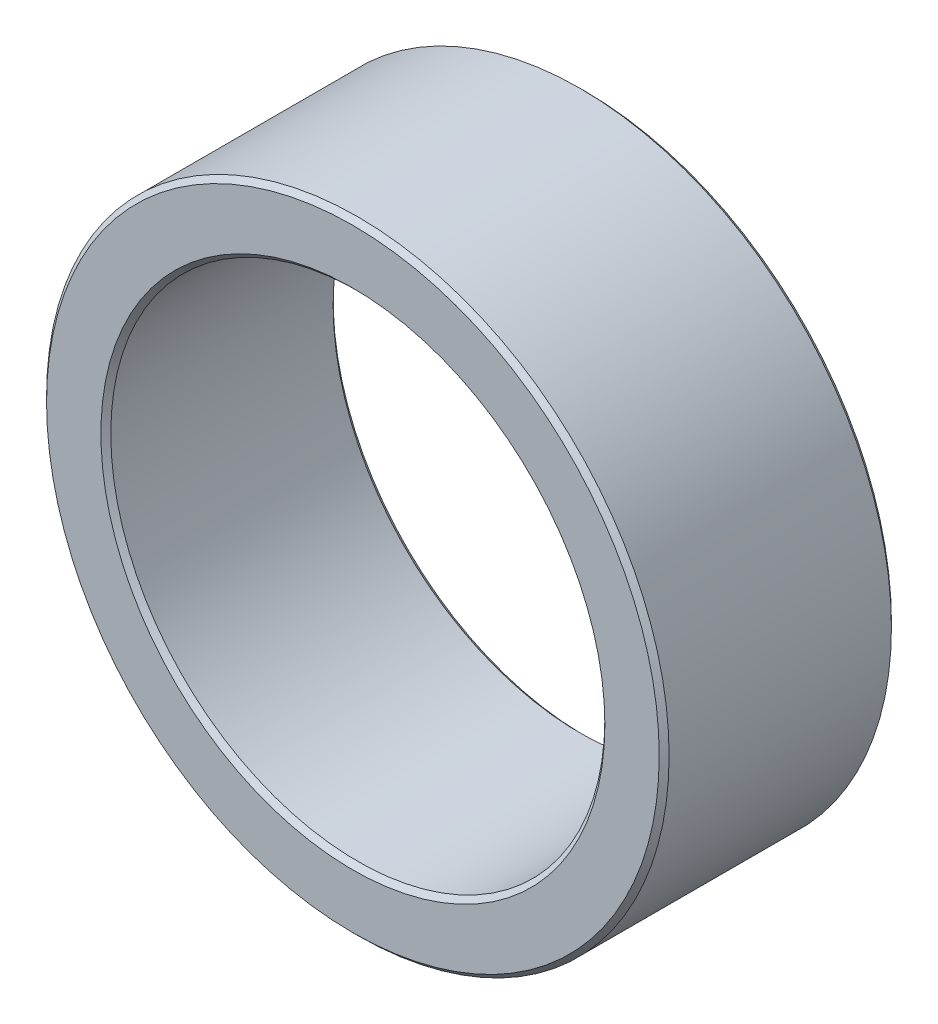
from build123d import *

# Parameters (mm, degrees)
SKETCH_1_R      = 31.5
SKETCH_1_R_2    = 25
EXTRUDE_1_DEPTH = 23.5
CHAMFER_1_SIZE  = 0.5


with BuildPart() as part:
    # 草图1 → 凸台-拉伸1 (new body)
    with BuildSketch(Plane.XY):
        Circle(SKETCH_1_R)
        Circle(SKETCH_1_R_2, mode=Mode.SUBTRACT)
    extrude(amount=EXTRUDE_1_DEPTH)

    # 倒角1
    chamfer_1_edges = [part.edges().sort_by_distance(p)[0] for p in [
        (-31.5, 0, 0),
        (-31.5, 0, 23.5),
        (-25, 0, 0),
        (-25, 0, 23.5),
    ]]
    chamfer(chamfer_1_edges, length=CHAMFER_1_SIZE)


solid = part.part
